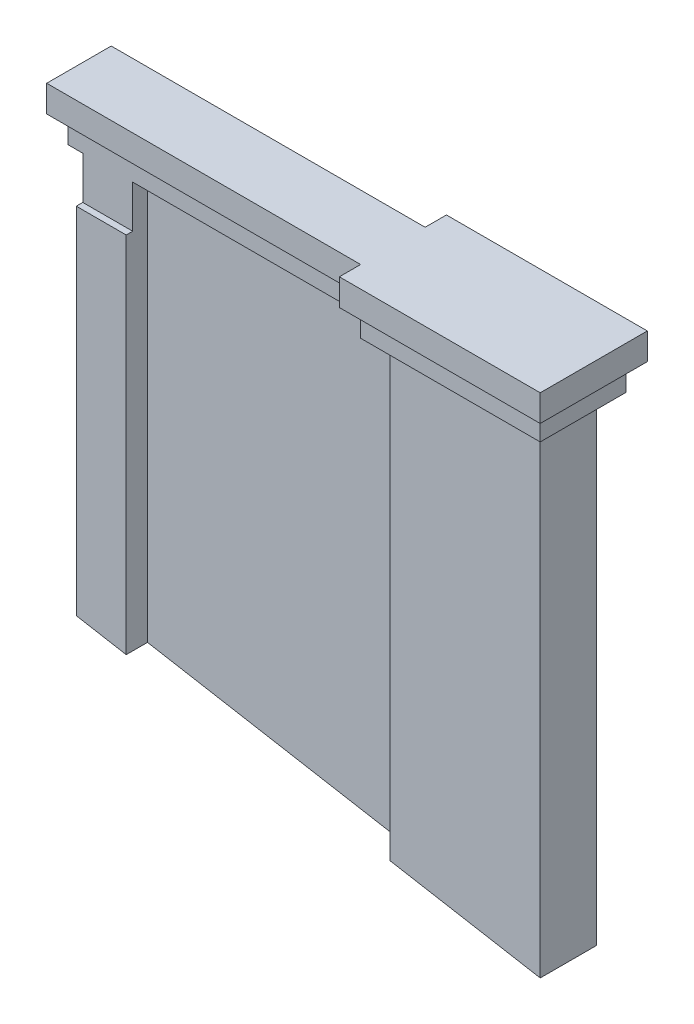
SolidWorks part; units mm, degrees
ref_plane "Front Plane" through (0, 0, 0) normal (0, 0, 1) x (1, 0, 0)
ref_plane "Top Plane" through (0, 0, 0) normal (0, 1, 0) x (1, 0, 0)
ref_plane "Right Plane" through (0, 0, 0) normal (1, 0, 0) x (0, 0, -1)
sketch "Sketch1" plane through (0, 0, 0) normal (0, 1, 0) x (1, 0, 0)
  line L11 (-43.58, 0) -> (-38.89, 0)
  line L12 (-38.89, 0) -> (-38.89, 2)
  line L13 (-14.09, 0) -> (0, 0)
  line L14 (-14.09, 2) -> (-14.09, 0)
  line L15 (-38.89, 2) -> (-14.09, 2)
  line L16 (-43.58, 3.28) -> (-43.58, 0)
  line L17 (-14.09, 3.28) -> (-43.58, 3.28)
  line L18 (-14.09, 5.28) -> (-14.09, 3.28)
  line L19 (0, 5.28) -> (-14.09, 5.28)
  line L20 (0, 0) -> (0, 5.28)
extrude "Boss-Extrude1" add sketch "Sketch1" along normal blind 45
sketch "Sketch2" plane through (0, 0, 0) normal (0, 0, 1) x (1, 0, 0)
  line L0 (0, 0) -> (-43.58, 0)
  line L1 (-43.58, 0) -> (-43.58, 7.6843)
  line L2 (-43.58, 45) -> (-43.58, 0) construction
  line L3 (-43.58, 7.6843) -> (0, 0)
  dimension "D1" = 10
extrude "Cut-Extrude1" cut sketch "Sketch2" against normal through all
sketch "Sketch3" plane through (0, 45, 0) normal (0, 1, 0) x (1, 0, 0)
  line L10 (-44.97, 4.67) -> (-44.97, 0.61)
  line L13 (-44.97, 0.61) -> (-15.48, 0.61)
  line L14 (-15.48, 0.61) -> (-15.48, -1.39)
  line L15 (-15.48, -1.39) -> (1.39, -1.39)
  line L16 (1.39, -1.39) -> (1.39, 6.67)
  line L17 (1.39, 6.67) -> (-15.48, 6.67)
  line L18 (-15.48, 6.67) -> (-15.48, 4.67)
  line L19 (-15.48, 4.67) -> (-44.97, 4.67)
extrude "Boss-Extrude2" add sketch "Sketch3" along normal blind 2.5
sketch "Sketch4" plane through (0, 47.5, 0) normal (0, 1, 0) x (1, 0, 0)
  line L10 (-45.97, 5.67) -> (-45.97, -0.39)
  line L13 (-45.97, -0.39) -> (-16.48, -0.39)
  line L14 (-16.48, -0.39) -> (-16.48, -2.39)
  line L15 (-16.48, -2.39) -> (2.39, -2.39)
  line L16 (2.39, -2.39) -> (2.39, 7.67)
  line L17 (2.39, 7.67) -> (-16.48, 7.67)
  line L18 (-16.48, 7.67) -> (-16.48, 5.67)
  line L19 (-16.48, 5.67) -> (-45.97, 5.67)
extrude "Boss-Extrude3" add sketch "Sketch4" along normal blind 2.5
sketch "Sketch5" plane through (-43.58, 0, 0) normal (-1, 0, 0) x (0, 0, 1)
  line L0 (-0.61, 45) -> (0, 45)
  line L1 (0, 45) -> (0, 41)
  line L2 (0, 45) -> (0, 7.6843) construction
  line L3 (-0.61, 45) -> (-0.61, 41)
  line L4 (-0.61, 41) -> (0, 41)
extrude "Cut-Extrude2" cut sketch "Sketch5" against normal blind 10
